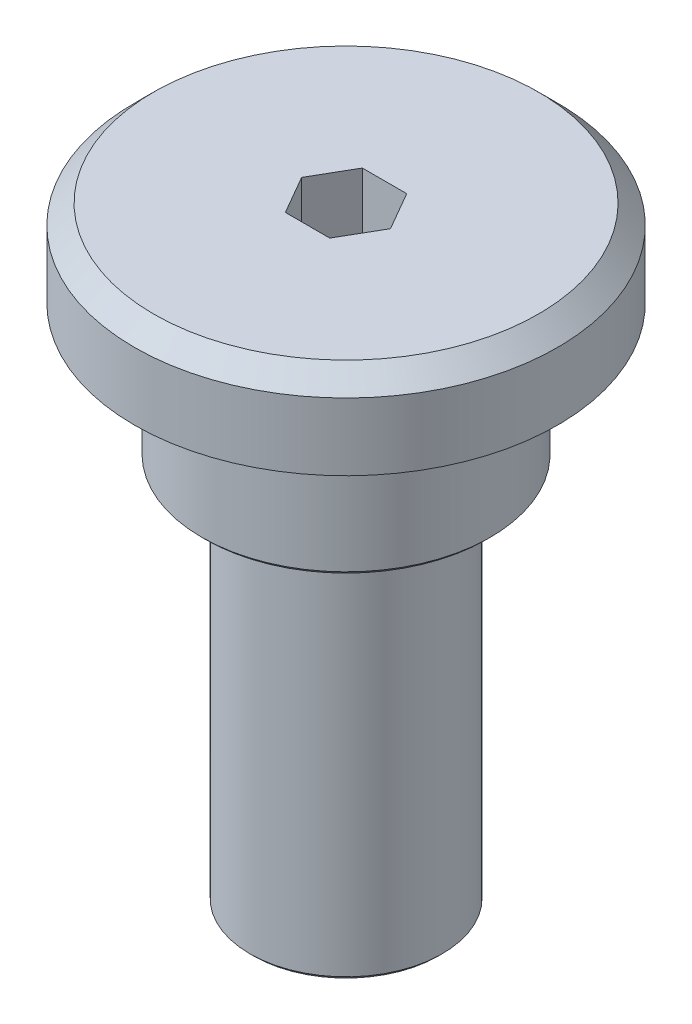
from build123d import *

# Parameters (mm, degrees)
SKETCH_1_R          = 5
EXTRUDE_1_DEPTH     = 20
SKETCH_2_R          = 7.5
EXTRUDE_2_DEPTH     = 7
SKETCH_3_R          = 11
EXTRUDE_3_DEPTH     = 4.5
CHAMFER_1_SIZE      = 1
CHAMFER_2_SIZE      = 0.2
CHAMFER_3_SIZE      = 0.2
CUT_EXTRUDE_1_DEPTH = 4


with BuildPart() as part:
    # 草图1 → 凸台-拉伸1 (new body)
    with BuildSketch(Plane(origin=(0, 0, 0), x_dir=(1, 0, 0), z_dir=(0, 1, 0))):
        with Locations(Location((0, 0, 0), (0, 0, 270))):
            Circle(SKETCH_1_R)
    extrude(amount=EXTRUDE_1_DEPTH)

    # 草图2 → 凸台-拉伸2 (add)
    with BuildSketch(Plane(origin=(0, 20, 0), x_dir=(1, 0, 0), z_dir=(0, 1, 0))):
        with Locations(Location((0, 0, 0), (0, 0, 270))):
            Circle(SKETCH_2_R)
    extrude(amount=EXTRUDE_2_DEPTH)

    # 草图3 → 凸台-拉伸3 (add)
    with BuildSketch(Plane(origin=(0, 27, 0), x_dir=(1, 0, 0), z_dir=(0, 1, 0))):
        with Locations(Location((0, 0, 0), (0, 0, 270))):
            Circle(SKETCH_3_R)
    extrude(amount=EXTRUDE_3_DEPTH)

    # 倒角1
    chamfer_1_edges = [part.edges().sort_by_distance(p)[0] for p in [
        (0, 31.5, -11),
    ]]
    chamfer(chamfer_1_edges, length=CHAMFER_1_SIZE)

    # 倒角2
    chamfer_2_edges = [part.edges().sort_by_distance(p)[0] for p in [
        (0, 20, -7.5),
    ]]
    chamfer(chamfer_2_edges, length=CHAMFER_2_SIZE)

    # 倒角3
    chamfer_3_edges = [part.edges().sort_by_distance(p)[0] for p in [
        (0, 0, -5),
    ]]
    chamfer(chamfer_3_edges, length=CHAMFER_3_SIZE)

    # 草图4 → 切除-拉伸1 (cut)
    with BuildSketch(Plane(origin=(0, 31.5, 0), x_dir=(1, 0, 0), z_dir=(0, 1, 0))):
        Polygon((2.309401077, 0), (1.154700538, 2), (-1.154700538, 2), (-2.309401077, 0), (-1.154700538, -2), (1.154700538, -2), align=None)
    extrude(amount=-CUT_EXTRUDE_1_DEPTH, mode=Mode.SUBTRACT)


solid = part.part
